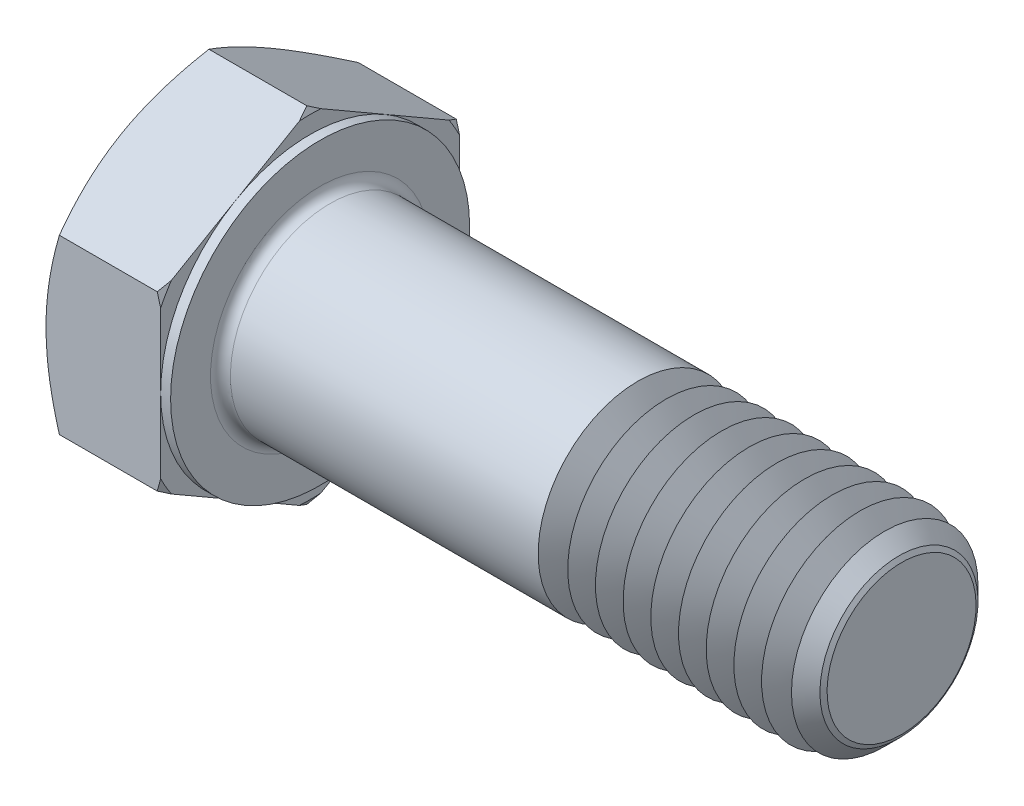
SolidWorks part; units mm, degrees
extrude "基体-拉伸" add sketch "草图1" along normal blind 7.5
sketch "草图1" plane through (0, 0, 0) normal (1, 0, 0) x (0, 0, -1)
  line L0 (9, 5.1962) -> (9, -5.1962)
  line L1 (-9, 5.1962) -> (-9, -5.1962)
  line L2 (9, -5.1962) -> (0, -10.3923)
  line L3 (0, -10.3923) -> (-9, -5.1962)
  line L4 (9, 5.1962) -> (0, 10.3923)
  line L5 (0, 10.3923) -> (-9, 5.1962)
revolve "切除-旋转1" cut sketch "草图3" angle 360 about L6
sketch "草图3" plane through (0, 0, 0) normal (0, 0, 1) x (1, 0, 0)
  line L0 (0, 9) -> (3.6906, 15.3923)
  line L1 (0, 10.3923) -> (0, 5.1962) construction
  line L2 (3.6906, 15.3923) -> (3.6906, 20.3923)
  line L3 (3.6906, 20.3923) -> (-10, 20.3923)
  line L4 (-10, 20.3923) -> (-10, 9)
  line L5 (-10, 9) -> (0, 9)
  line L6 (0, 0) -> (99.06, 0) construction
  line L7 (7.5, 10.3923) -> (0, 10.3923) construction
material "5.6级"
ref_plane "前视" through (0, 0, 0) normal (0, 0, 1) x (1, 0, 0)
ref_plane "上视" through (0, 0, 0) normal (0, 1, 0) x (1, 0, 0)
ref_plane "右视" through (0, 0, 0) normal (1, 0, 0) x (0, 0, -1)
sketch "草图2" plane through (0, 0, 0) normal (0, 0, 1) x (1, 0, 0)
  line L0 (0, 5.1962) -> (0, -5.1962) construction
  line L1 (0, 0) -> (42.5, 0)
  line L2 (0, 0) -> (0, 6)
  line L3 (0, 6) -> (7.7917, 6)
  line L4 (42.5, 0) -> (42.5, 4.4845)
  line L5 (7.5, 10.3923) -> (7.5, 5.1962) construction
  line L7 (0, 0) -> (96.52, 0) construction
  line L8 (42.5, -4.4845) -> (7.7917, -6) construction
  line L9 (0, -6) -> (7.7917, -6) construction
  line L10 (9.25, 15.24) -> (9.25, -1.27) construction
  line L11 (27.5, 15.24) -> (27.5, -1.27) construction
  line L12 (7.5, 5.1962) -> (7.5, -5.1962) construction
  line L13 (7.7917, 6) -> (42.5, 6)
  line L14 (42.5, 6) -> (42.5, 4.4845)
revolve "凸台-旋转1" add sketch "草图2" angle 360 about L7
cosmetic thread "螺旋线1" parameters "Thread_length"=15, "Thread_minor"=8.969
sketch "草图5" plane through (0, 0, 0) normal (0, 0, 1) x (1, 0, 0)
  line L0 (7.5, 9) -> (3.8094, 15.3923)
  line L1 (7.5, 10.3923) -> (7.5, 5.1962) construction
  line L2 (3.8094, 15.3923) -> (3.8094, 20.3923)
  line L3 (3.8094, 20.3923) -> (13.8094, 20.3923)
  line L4 (13.8094, 20.3923) -> (13.8094, 9)
  line L5 (13.8094, 9) -> (7.5, 9)
  line L7 (7.5, 10.3923) -> (0.8038, 10.3923) construction
  line L8 (0, 0) -> (99.06, 0) construction
  line L9 (0, 0) -> (99.06, 0) construction
revolve "切除-旋转2" cut sketch "草图5" angle 360 about L8
sketch "草图4" plane through (0, 0, 0) normal (0, 0, 1) x (1, 0, 0)
  line L1 (7.5, 10.3923) -> (7.5, 5.1962) construction
  line L2 (7.5, 9) -> (6.9, 9)
  line L3 (7.5, 9) -> (7.5, 20.3923)
  line L4 (7.5, 20.3923) -> (6.9, 20.3923)
  line L5 (0, 0) -> (95.25, 0) construction
  line L6 (0, 0) -> (96.52, 0) construction
  line L7 (6.9, 9) -> (6.9, 20.3923)
  line L8 (6.6962, 10.3923) -> (0.8038, 10.3923) construction
revolve "切除-旋转3" cut sketch "草图4" angle 360 about L5
chamfer "倒角" distance 1.4 angle 45 1 edges at (42.5, 0, 6)
fillet "圆角" radius 0.6 1 edges at (7.5, 0, -6)
sketch "草图6" plane through (0, 0, 0) normal (0, 0, 1) x (1, 0, 0)
  line L0 (27.5, -4.4845) -> (26.625, -6)
  line L1 (27.5, -4.4845) -> (28.375, -6)
  line L2 (28.375, -6) -> (28.375, -7.5)
  line L3 (-3.175, 0) -> (5.1513, 0) construction
  line L5 (28.375, -7.5) -> (26.625, -7.5)
  line L6 (26.625, -7.5) -> (26.625, -6)
revolve "切除-旋转4" cut sketch "草图6" angle 360 about L3
pattern_linear "阵列(线性)1" count 10 spacing 1.6667 along (1, 0, 0) of "切除-旋转4"
equation "\"D3@草图1\" = \"s@草图1\" / 2"
equation "\"D4@草图1\" = \"D3@草图1\""
equation "\"D5@草图1\" = \"D4@草图1\""
equation "\"Thread_minor@螺旋线1\" = \"Minor_dia@草图2\""
equation "\"D1@草图3\" = \"s@草图1\" / 2"
equation "\"D1@草图5\" = \"s@草图1\" / 2"
equation "\"Head_ch_ang@草图5\" = \"Head_ch_ang@草图3\""
equation "\"D1@草图4\" = \"s@草图1\""
equation "\"Thread_length@螺旋线1\" = ((sgn( (\"l@草图2\" - \"p@草图2\" ) - \"h@草图2\" )-1)*( (\"l@草图2\" - \"p@草图2\" ) - \"h@草图2\" ))/-2+ \"h@草图2\""
equation "\"Thread_minor@草图6\" = \"Minor_dia@草图2\""
equation "\"Diameter@草图6\" = \"m@草图2\""
equation "\"Overcut@草图6\" = \"m@草图2\" * 1.25"
equation "\"Start@草图6\" = \"k@基体-拉伸\" + \"l@草图2\" - \"Thread_length@螺旋线1\"  '---Non-countersunk---"
equation "\"Num_threads@阵列(线性)1\" = int( \"Thread_length@螺旋线1\" / \"p@草图2\" + 0.999 )  + 1"
equation "\"Advance@阵列(线性)1\" = \"Thread_length@螺旋线1\" /  (\"Num_threads@阵列(线性)1\" - 1) 'relax it"
equation "\"Num_threads@阵列(线性)1\" = \"Num_threads@阵列(线性)1\" - sgn( \"Num_threads@阵列(线性)1\" - 1) '---chamfered tips only---"
equation "\"Minor_dia@草图2\" = \"m@草图2\"-\"p@草图2\" * 1.732"
equation "\"D1@倒角\" = \"p@草图2\"*0.8"
